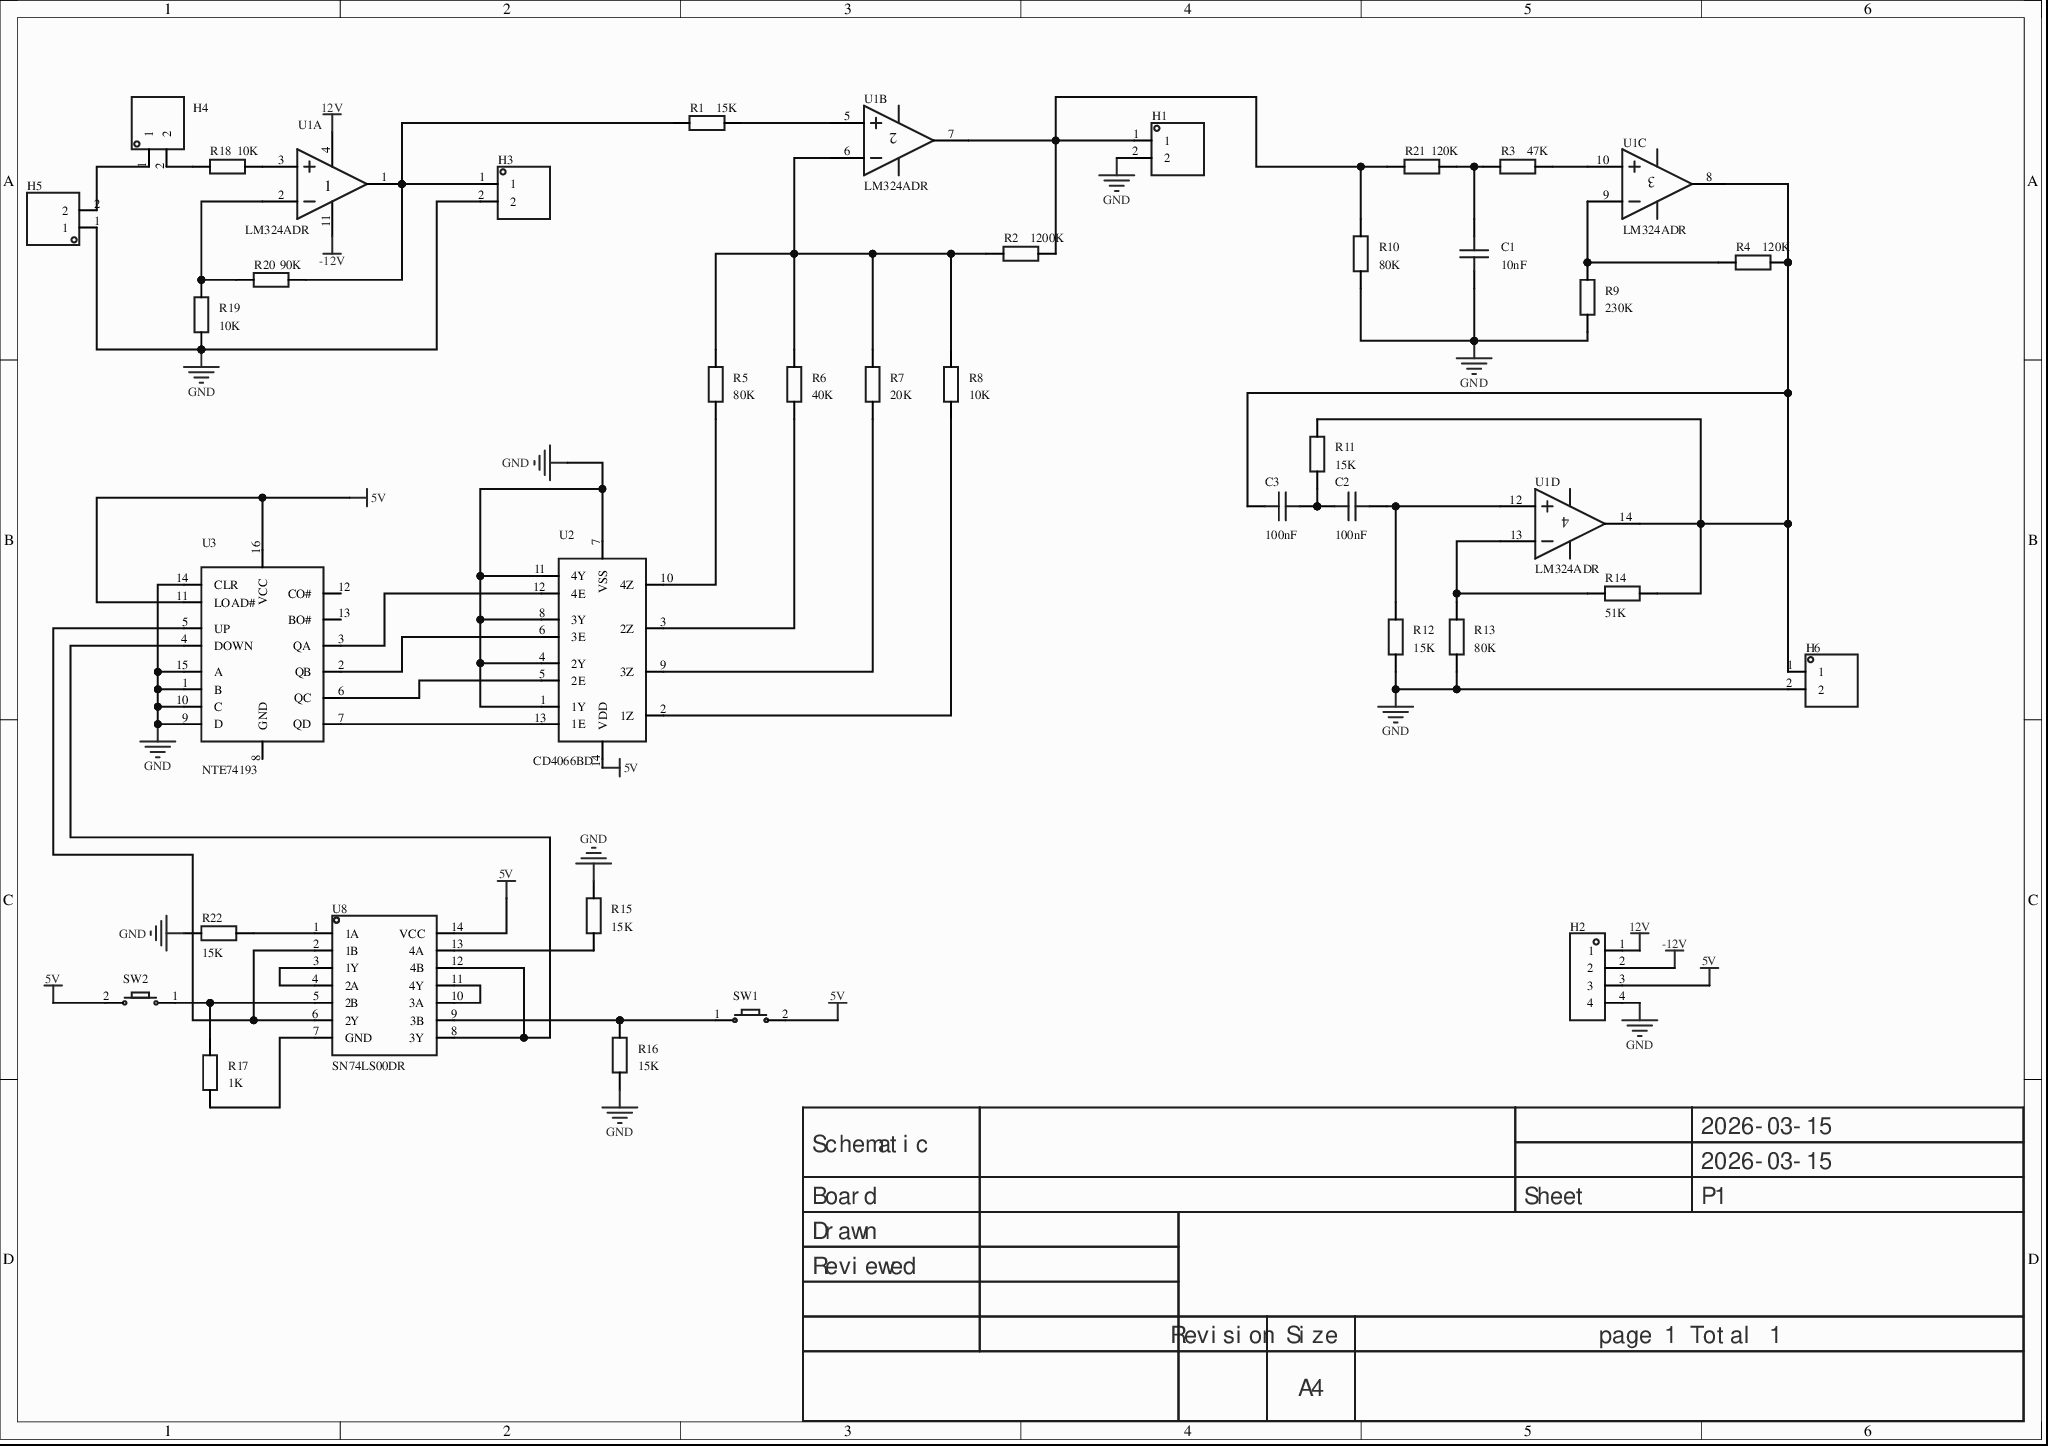
[diagram p0: MISC52000-3.schdoc]
# Altium project MISC52000-2.PrjPcb
1 sheet, 37 parts. Net scope: global (net labels, ports and power ports of the same name join across sheets).
Board file: MISC52000.pcbdoc

## Sheet MISC52000-3.schdoc
size 297 x 209 mm; Version: V1.0; @Project Name: MISC52000; @Update Date: 2026-03-15; @Create Date: 2026-03-15; @Board Name: MISC52000; @Create Time: 16:23:48; @Page Count: 1; @Page No: 1; @Schematic Name: MISC52000; @Update Time: 16:23:48; Size: A4

### Parts
C1  10nF  [C0603]
C2  100nF  [C0603]
C3  100nF  [C0603]
H1  (no value)  [HDR-TH_2P-P2.54-V-M-1]
H2  (no value)  [HDR-TH_4P-P2.54-V-M]
H3  (no value)  [HDR-TH_2P-P2.54-V-M-1]
H4  (no value)  [HDR-TH_2P-P2.54-V-M-1]
H5  (no value)  [HDR-TH_2P-P2.54-V-M-1]
H6  (no value)  [HDR-TH_2P-P2.54-V-M-1]
R1  15K  [R0603]
R2  1200K  [R0603]
R3  47K  [R0603]
R4  120K  [R0603]
R5  80K  [R0603]
R6  40K  [R0603]
R7  20K  [R0603]
R8  10K  [R0603]
R9  230K  [R0603]
R10  80K  [R0603]
R11  15K  [R0603]
R12  15K  [R0603]
R13  80K  [R0603]
R14  51K  [R0603]
R15  15K  [R0603]
R16  15K  [R0603]
R17  1K  [R0603]
R18  10K  [R0603]
R19  10K  [R0603]
R20  90K  [R0603]
R21  120K  [R0603]
R22  15K  [R0603]
SW1  (no value)  [Key_SMD_3x4x2]
SW2  (no value)  [Key_SMD_3x4x2]
U1  LM324ADR  [SOP-14_L8.6-W3.9-P1.27-LS6.0-BL]  (parts A,B,C,D of 4)
U2  CD4066BD  [SOP-14_L8.6-W3.9-P1.27-LS6.0-BL]
U3  NTE74193  [PDIP-16_L19.7-W6.6-P2.54-LS7.6-BL]
U8  SN74LS00DR  [SOIC-14_L8.7-W3.9-P1.27-LS6.0-BL]

### Nets
5V: H2.3 SW1.2 SW2.2 U2.14(VDD) U3.11(LOAD#) U3.16(VCC) U8.14(VCC)
12V: H2.1 U1.4(VCC)
-12V: H2.2 U1.11(GND)
GND: C1.1 H1.2 H2.4 H3.2 H5.1 H6.2 R9.1 R10.1 R12.1 R13.1 R15.2 R16.1 R19.1 R22.2 U2.1(1Y) U2.4(2Y) U2.7(VSS) U2.8(3Y) U2.11(4Y) U3.1(B) U3.9(D) U3.10(C) U3.14(CLR) U3.15(A)
NetC1_2: C1.2 R3.1 R21.2
NetC2_1: C2.1 R12.2 U1.12(4IN+)
NetC2_2: C2.2 C3.1 R11.1
NetC3_2: C3.2 H6.1 R4.2 R11.2 R14.1 U1.8(3OUT) U1.14(4OUT)
NetH1_1: H1.1 R2.2 R10.2 R21.1 U1.7(2OUT)
NetH3_1: H3.1 R1.1 R20.2 U1.1(1OUT)
NetH4_1: H4.1 H5.2
NetH4_2: H4.2 R18.1
NetR1_2: R1.2 U1.5(2IN+)
NetR2_1: R2.1 R5.2 R6.2 R7.2 R8.2 U1.6(2IN-)
NetR3_2: R3.2 U1.10(3IN+)
NetR4_1: R4.1 R9.2 U1.9(3IN-)
NetR5_1: R5.1 U2.10(4Z)
NetR6_1: R6.1 U2.3(2Z)
NetR7_1: R7.1 U2.9(3Z)
NetR8_1: R8.1 U2.2(1Z)
NetR13_2: R13.2 R14.2 U1.13(4IN-)
NetR15_1: R15.1 U8.13(4A)
NetR16_2: R16.2 SW1.1 U8.9(3B)
NetR17_1: R17.1 U8.7(GND)
NetR17_2: R17.2 SW2.1 U8.5(2B)
NetR18_2: R18.2 U1.3(1IN-)
NetR19_2: R19.2 R20.1 U1.2(1IN+)
NetR22_1: R22.1 U8.1(1A)
NetU2_5: U2.5(2E) U3.6(QC)
NetU2_6: U2.6(3E) U3.2(QB)
NetU2_12: U2.12(4E) U3.3(QA)
NetU2_13: U2.13(1E) U3.7(QD)
NetU3_4: U3.4(DOWN) U8.8(3Y) U8.12(4B)
NetU3_5: U3.5(UP) U8.2(1B) U8.6(2Y)
NetU8_3: U8.3(1Y) U8.4(2A)
NetU8_10: U8.10(3A) U8.11(4Y)

Not connected (* = marked no-connect by the designer): U3 8(GND) 12(CO#) 13(BO#)

### Notes on the sheet
- 2026-03-15
- Schematic
- Board
- Sheet
- P1
- Drawn
- Reviewed
- Revision
- Size
- A4
- page 1 Total 1

### Library data of the parts
C1-C3 = CAP_0603: Symbol: Capacitance; 3D Model: ac125912035d415993ca9572d50418b10819f05c4eef4c71ace90d822a990e87; 3D Model Transform: 62.992,31.496,0,0,0,0,0,0,0; ConvertToPcb: yes; ModelName: C0603_L1.6-W0.8-H0.8; Device: CAP_0603; Supplier Footprint: 0603; AddInBom: yes; FootprintName: C0603
  C1: Value: 10nF
  C2 C3: Value: 100nF
H1 H3-H6 = HDR-M_2.54_1x2P: Symbol: 210S-1*2P L=11.6MMGold-plated black; 3D Model: 79b2e9f2d70a4d68a1b7098f27c6d4c50819f05c4eef4c71ace90d822a990e87; 3D Model Transform: 200,100,0,0,0,0,0,0,-118.11; ConvertToPcb: yes; ModelName: HDR-M-2.54_1x2; Device: HDR-M_2.54_1x2P; Supplier Part: C124375; Supplier Footprint: 插件; AddInBom: yes; FootprintName: HDR-TH_2P-P2.54-V-M-1
H2 = HDR-M_2.54_1x4P: Symbol: PZ254V-11-04P; ConvertToPcb: yes; ModelId: 112f4d05e8d64e99ab9a333894bea4f90819f05c4eef4c71ace90d822a990e87; ModelName: HDR-TH_4P-P2.54-M-LI-1X4P; ModelTransform: 399.999,104.7242,0,0,0,0,0,0,-118.11; Device: HDR-M_2.54_1x4P; AddInBom: yes; SupplierPart: C492403; Supplier Footprint: 插件; FootprintName: HDR-TH_4P-P2.54-V-M
R1-R22 = Res_0603: Symbol: Resistor; 3D Model: fc143cca1e79419f9cd78b61e9279f080819f05c4eef4c71ace90d822a990e87; 3D Model Transform: 31.8897,63.7794,0,90,0,0,0,0,0; ConvertToPcb: yes; Device: Res_0603; Supplier Footprint: 0603; AddInBom: yes; FootprintName: R0603; ModelName: R0603
  R1 R11 R12 R15 R16 R22: Value: 15K
  R2: Value: 1200K
  R3: Value: 47K
  R4 R21: Value: 120K
  R5 R10 R13: Value: 80K
  R6: Value: 40K
  R7: Value: 20K
  R8 R18 R19: Value: 10K
  R9: Value: 230K
  R14: Value: 51K
  R17: Value: 1K
  R20: Value: 90K
SW1 SW2 = Key_SMD_3x4x2: Symbol: Tact switch x2; ConvertToPcb: yes; ModelId: 63599cce708d48afbce1b0db003544770819f05c4eef4c71ace90d822a990e87; ModelName: SW-SMD_L4.0-W2.9-H2-LS5.0; ModelTransform: 196.85,114.17,79.13,0,0,0,0,0,0; Device: Key_SMD_3x4x2; AddInBom: yes; Supplier Footprint: SMD; FootprintName: Key_SMD_3x4x2
U1 = LM324ADR_C2837469: Amplifiers: four; Rail-to-rail: -; Gain bandwidth product (GBP): -; Input offset voltage (Vos): 9mV; Input bias current (Ib): 250nA;; Manufacturer: UMW(友台半导体); Relevance: []; 3D Model: 520b569c4a2341089bdfdd9bf52b86190819f05c4eef4c71ace90d822a990e87; 3D Model Transform: 339.763,236.22,0,0,0,0,0,0,0; Input Offset Voltage Drift(Vos TC): 7uV/℃; Common Mode Rejection Ratio(CMRR): 80dB; AddInBom: yes; Symbol: LM324ADR_C2837469; Device: LM324ADR_C2837469; LCSC Part Name: LM324ADR; Supplier Part: C2837469; Manufacturer Part: LM324ADR; Supplier Footprint: SOP-14; JLCPCB Part Class: Extended Part; Supplier: LCSC; Number of Channels: Four; Rail to Rail: -; Gain Bandwidth Product: -; Vos - Input Offset Voltage: 9mV; Ib - Input Bias Current: 250nA; Input Offset Current(Ios): -; Input offset current drift(Ios TC): -; Quiescent Current: -; Output Current: -; Operating Temperature: -40℃~+85℃; ConvertToPcb: yes; FootprintName: SOP-14_L8.6-W3.9-P1.27-LS6.0-BL; ModelName: SOP-14_L8.6-W3.9-P1.27-LS6.0-BL
U2 = CD4066BD: Switch circuit: -; On-resistance (Ron): 1.05kΩ;; Manufacturer: HTC; 3D Model: 520b569c4a2341089bdfdd9bf52b86190819f05c4eef4c71ace90d822a990e87; 3D Model Transform: 339.763,236.22,0,0,0,0,0,0,0; Voltage - Supply: 3V~18V; Con: 7.5pF; Bandwidth: 40MHz; Propagation Delay (tpd): 40ns; AddInBom: yes; Symbol: CD4066BD; Device: CD4066BD; LCSC Part Name: CD4066BD; Supplier Part: C558790; Manufacturer Part: CD4066BD; Supplier Footprint: SOP-14; JLCPCB Part Class: Extended Part; Supplier: LCSC; Switch Circuit: -; Ron: 1.05kΩ; Operating Temperature: -55℃~+125℃; ConvertToPcb: yes; FootprintName: SOP-14_L8.6-W3.9-P1.27-LS6.0-BL; ModelName: SOP-14_L8.6-W3.9-P1.27-LS6.0-BL
U3 = NTE74193: Operating voltage: -; Number of elements: 1; Count rate: 32MHz;; Manufacturer: NTE ELECTRONICS, INC.; 3D Model: 60304d8eb9b246fdb135cb3d16f241a80819f05c4eef4c71ace90d822a990e87; 3D Model Transform: 787.4,311.8104,0,0,0,0,0,0,-118.11; Logic Type: Divide-by-2; Direction: Down counter; Up counter; Number of Elements: 1; Reset: Asynchronous; Timing: Synchronous; AddInBom: yes; ModelName: PDIP-16_L19.7-W6.6-H5.1-P2.54-LS7.6-BL; Symbol: NTE74193; Device: NTE74193; LCSC Part Name: NTE74193; Supplier Part: C6345915; Manufacturer Part: NTE74193; Supplier Footprint: PDIP-16; JLCPCB Part Class: Extended Part; Supplier: LCSC; Voltage - Supply: -; Count Rate: 32MHz; Operating Temperature: 0℃~+70℃; ConvertToPcb: yes; FootprintName: PDIP-16_L19.7-W6.6-P2.54-LS7.6-BL
U8 = SN74LS00DR: Logic type: NAND gate; Channels: 4; Operating voltage: 4.75V~5.25V; Propagation delay (tpd): 15ns@5V,15pF;; Manufacturer: TI(德州仪器); AddInBom: yes; ModelId: 8dbf5b715d42428c85558507ae5a252b0819f05c4eef4c71ace90d822a990e87; ModelName: SOIC-14_L8.6-W3.9-H1.8-LS6.0-P1.27; ModelTransform: 338.583,236.22,0,0,0,0,0,0.001,0; Number of Channels: 4; Current - Output Low(IOL): 8mA; Current - Output High(IOH): 400uA; Input Logic Level - High: 2V; Input Logic Level - Low: 800mV; Output Logic Level - High: 2.5V; Output Logic Level - Low: 500mV; Input Number: 2; Symbol: SN74LS00DR; Device: SN74LS00DR; LCSC Part Name: 四路 2 输入正与非门; SupplierPart: C74558; ManufacturerPart: SN74LS00DR; Supplier Footprint: SOIC-14; JLCPCB Part Class: Extended Part; Supplier: LCSC; ConvertToPcb: yes; FootprintName: SOIC-14_L8.7-W3.9-P1.27-LS6.0-BL; Logic Type: NAND gate; Voltage - Supply: 4.75V~5.25V; Series: 74LS series; Propagation Delay: 15ns@5V,15pF; Operating Temperature: 0℃~+70℃